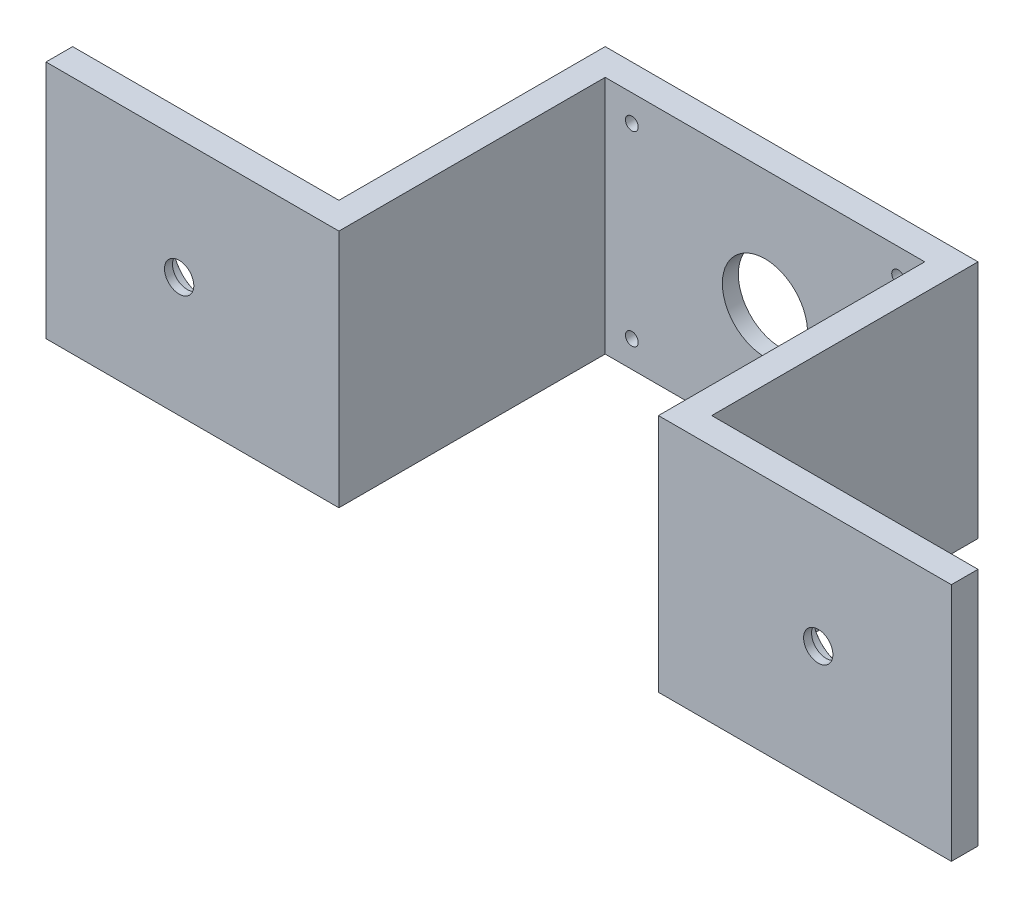
SolidWorks part; units mm, degrees
ref_plane "Front Plane" through (0, 0, 0) normal (0, 0, 1) x (1, 0, 0)
ref_plane "Top Plane" through (0, 0, 0) normal (0, 1, 0) x (1, 0, 0)
ref_plane "Right Plane" through (0, 0, 0) normal (1, 0, 0) x (0, 0, -1)
sketch "Sketch7" plane through (0, 0, 0) normal (0, 1, 0) x (1, 0, 0)
  line L0 (0, 0) -> (55, 0)
  line L1 (55, 0) -> (55, 50)
  line L2 (55, 50) -> (115, 50)
  line L3 (115, 50) -> (115, 0)
  line L4 (115, 0) -> (170, 0)
  line L5 (170, 0) -> (170, 5)
  line L6 (170, 5) -> (120, 5)
  line L7 (120, 5) -> (120, 55)
  line L8 (120, 55) -> (50, 55)
  line L9 (50, 55) -> (50, 5)
  line L10 (50, 5) -> (0, 5)
  line L11 (0, 5) -> (0, 0)
  dimension "D1" = 55
  dimension "D2" = 60
  dimension "D3" = 55
  dimension "D4" = 5
  dimension "D5" = 5
  dimension "D6" = 70
  dimension "D7" = 5
  dimension "D8" = 5
  dimension "D9" = 50
extrude "Boss-Extrude3" add sketch "Sketch7" along normal blind 45
sketch "Sketch8" plane through (0, 0, -5) normal (0, 0, -1) x (-1, 0, 0)
  line L0 (-170, 45) -> (-120, 0) construction
  line L2 (-50, 45) -> (0, 0) construction
hole_wizard "CBORE for M5 Hex Cap Screw1" positions "Sketch9" profile "Sketch10" counterbore size "M5" standard "ISO" end condition through all
sketch "Sketch9" plane through (0, 0, -5) normal (0, 0, -1) x (-1, 0, 0)
  line L0 (-170, 45) -> (-120, 0) construction
  line L1 (-50, 45) -> (0, 0) construction
  point P0 (-145, 22.5)
  point P4 (-25, 22.5)
sketch "Sketch10" plane through (145, 22.5, -5) normal (1, 0, 0) x (0, 1, 0)
  line L0 (0, 0) -> (0, 5)
  line L1 (0, 5) -> (2.75, 5)
  line L3 (2.75, 5) -> (2.75, 3.5)
  line L4 (6.119, 3.5) -> (2.75, 3.5)
  line L5 (6.119, 3.5) -> (6.119, 0.025)
  line L6 (6.119, 0.025) -> (6.144, 0)
  line L7 (6.144, 0) -> (0, 0)
  line L8 (-6.119, 0.025) -> (-6.144, 0) construction
  line L11 (0, -6.35) -> (0, 107.95) construction
  dimension "通孔孔直径" = 5.5
  dimension "通孔孔深度" = 5
  dimension "柱形沉头孔直径" = 12.238
  dimension "柱形沉头孔深度" = 3.5
  dimension "近端锥形沉头孔直径" = 12.288
  dimension "近端锥形沉头孔角度" = 90
sketch "Sketch11" plane through (0, 0, -5) normal (0, 0, -1) x (-1, 0, 0)
  circle A0 centre (-145, 22.5) radius 2.75
sketch "Sketch12" plane through (0, 0, -55) normal (0, 0, -1) x (-1, 0, 0)
  line L0 (-120, 45) -> (-50, 0)
  line L1 (-170, 45) -> (-120, 45) construction
  line L2 (-120, 45) -> (-120, 0) construction
  line L3 (-50, 45) -> (-50, 0) construction
  line L4 (-120, 0) -> (-50, 0) construction
  circle A0 centre (-85, 22.5) radius 8
extrude "Cut-Extrude1" cut sketch "Sketch12" against normal blind 10 contours L0 A0 | L0 A0
sketch "Sketch13" plane through (0, 0, -55) normal (0, 0, -1) x (-1, 0, 0)
  circle A0 centre (-85, 22.5) radius 15
extrude "Cut-Extrude2" cut sketch "Sketch13" against normal blind 2
sketch "Sketch14" plane through (0, 0, -55) normal (0, 0, -1) x (-1, 0, 0)
  circle A0 centre (-60, 5) radius 1.2043
  circle A1 centre (-60, 40) radius 1.2
  circle A2 centre (-110, 5) radius 1.2
  circle A3 centre (-110, 40) radius 1.2
extrude "Cut-Extrude3" cut sketch "Sketch14" against normal blind 5
